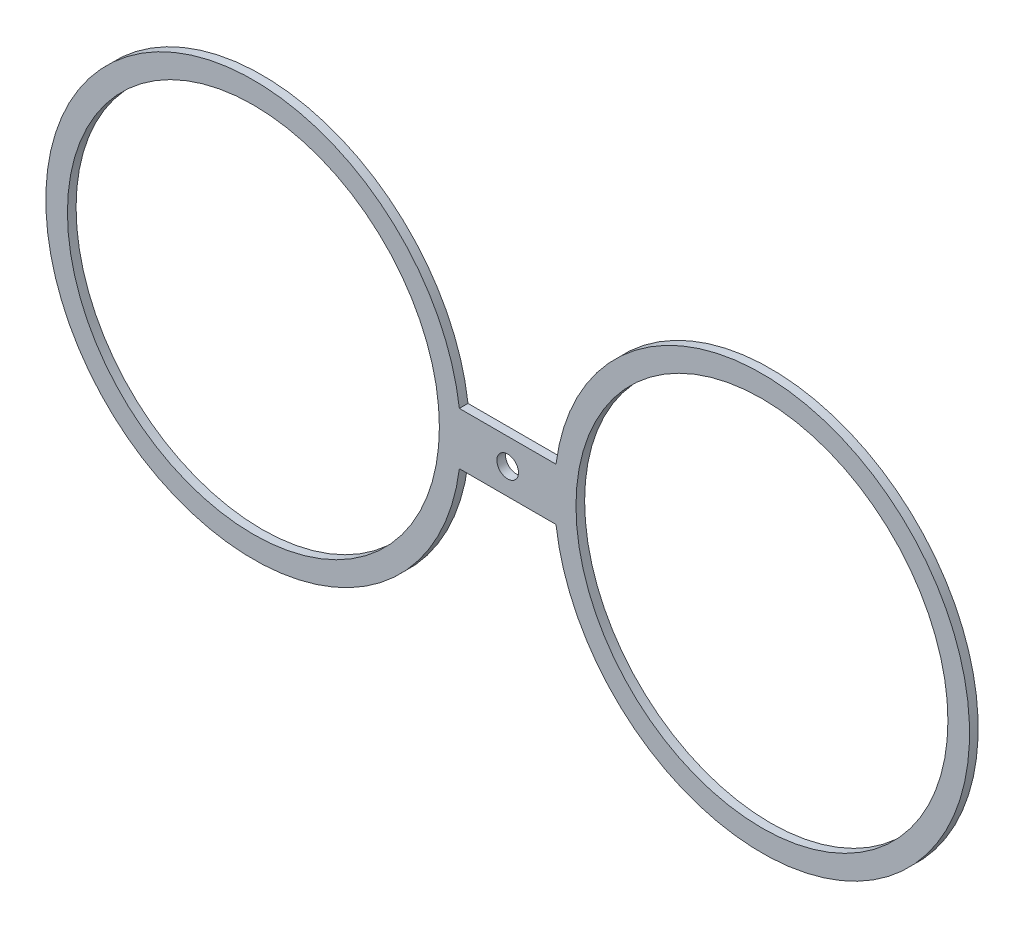
SolidWorks part; units mm, degrees
ref_plane "Front Plane" through (0, 0, 0) normal (0, 0, 1) x (1, 0, 0)
ref_plane "Top Plane" through (0, 0, 0) normal (0, 1, 0) x (1, 0, 0)
ref_plane "Right Plane" through (0, 0, 0) normal (1, 0, 0) x (0, 0, -1)
sketch "Sketch1" plane through (0, 0, 0) normal (0, 0, 1) x (1, 0, 0)
  line L0 (0, 0) -> (117.58, 0) construction
  line L5 (47.6178, 6.0452) -> (69.9622, 6.0452)
  line L6 (69.9591, -6.0204) -> (47.6209, -6.0204)
  circle A0 centre (0, 0) radius 43
  circle A1 centre (117.58, 0) radius 43
  circle A2 centre (58.79, 0) radius 2.5
  arc A3 (47.6178, 6.0452) -> (47.6209, -6.0204) centre (0, 0) ccw
  arc A4 (69.9591, -6.0204) -> (69.9622, 6.0452) centre (117.58, 0) ccw
  circle A5 centre (117.58, 0) radius 48 construction
  circle A6 centre (0, 0) radius 48 construction
  dimension "D1" = 117.58
  dimension "D2" = 86
  dimension "D3" = 86
  dimension "D4" = 5
  dimension "D5" = 5
  dimension "D6" = 5
extrude "Boss-Extrude1" add sketch "Sketch1" along normal blind 2
